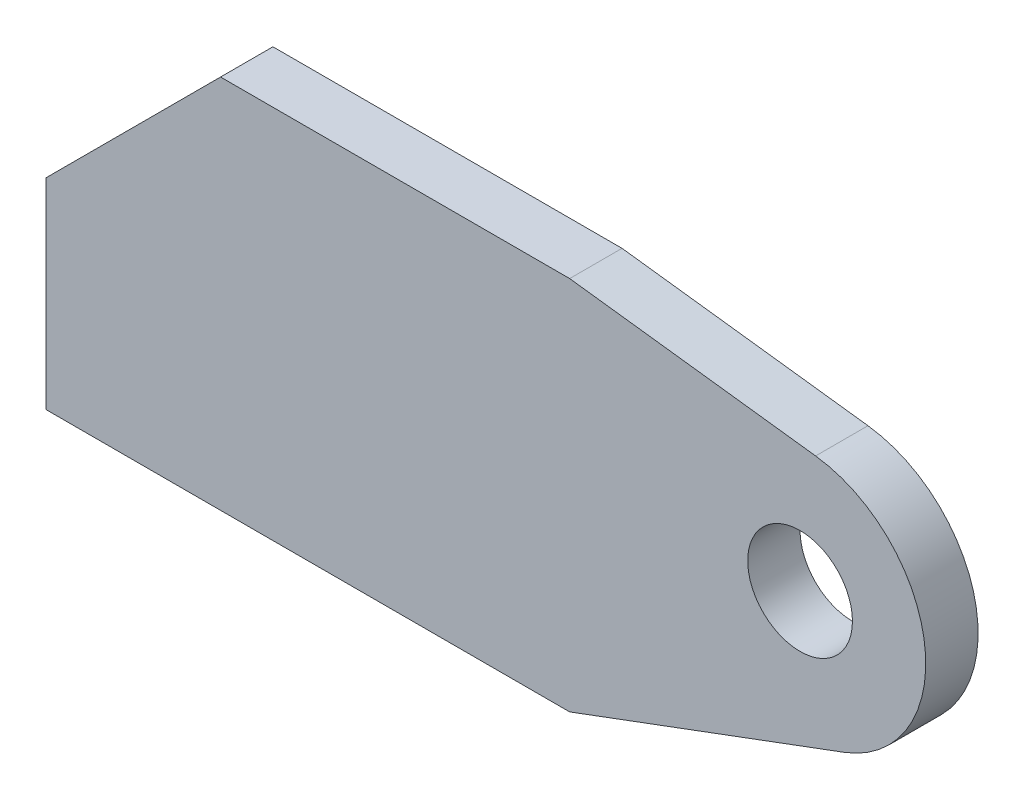
SolidWorks part; units mm, degrees
material "Q235"
ref_plane "Front Plane" through (0, 0, 0) normal (0, 0, 1) x (1, 0, 0)
ref_plane "Top Plane" through (0, 0, 0) normal (0, 1, 0) x (1, 0, 0)
ref_plane "Right Plane" through (0, 0, 0) normal (1, 0, 0) x (0, 0, -1)
sketch "Sketch1" plane through (0, 0, 0) normal (0, 0, 1) x (1, 0, 0)
  line L0 (0, 0) -> (300, 0)
  line L1 (300, 0) -> (457.1318, 58.5286)
  line L2 (440.9004, 197.4478) -> (300, 215)
  line L3 (300, 215) -> (100, 215)
  line L4 (100, 215) -> (0, 115)
  line L5 (0, 115) -> (0, 0)
  arc A0 (457.1318, 58.5286) -> (440.9004, 197.4478) centre (432, 126) ccw
  circle A1 centre (432, 126) radius 30
  dimension "D5" = 72
  dimension "D8" = 126
  dimension "D9" = 60
  dimension "D1" = 215
  dimension "D2" = 100
  dimension "D3" = 100
  dimension "D4" = 432
  dimension "D6" = 300
  dimension "D7" = 300
extrude "Boss-Extrude1" add sketch "Sketch1" along normal blind 30
